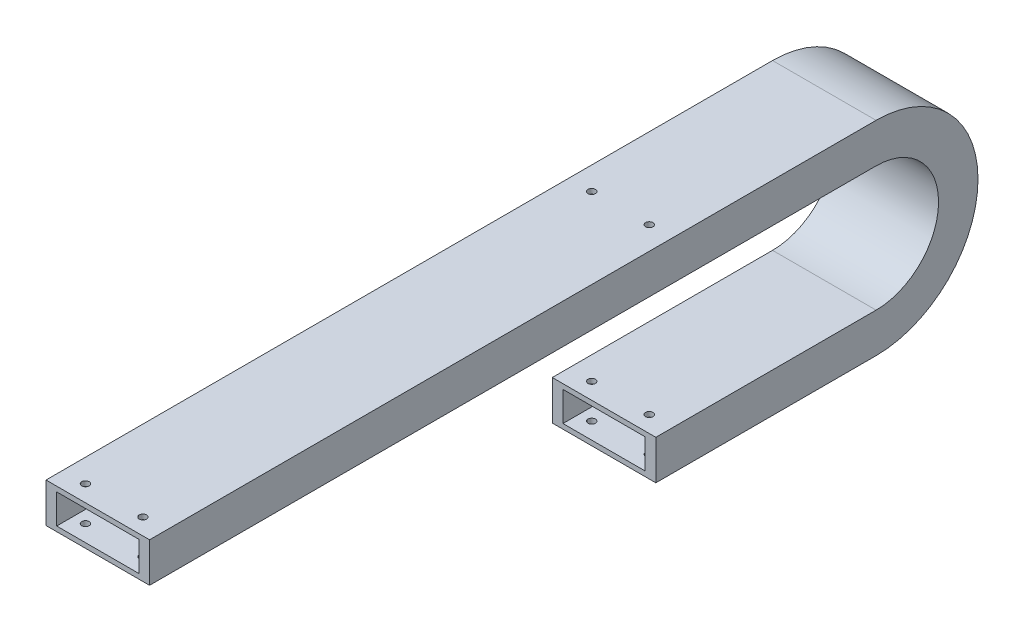
from build123d import *

# Parameters (mm, degrees)
SKETCH_1_W          = 63
SKETCH_1_H          = 24
SKETCH_1_W_2        = 50
SKETCH_1_H_2        = 18
SKETCH_5_R          = 2.25
CUT_EXTRUDE_3_DEPTH = 334.514992167


with BuildPart() as part:
    # 扫描1: sweep along a path in 草图2
    with BuildLine(Plane(origin=(0, 0, 0), x_dir=(0, 0, -1), z_dir=(1, 0, 0))) as sweep_1_path:
        Line((0, 0), (134, 0))
        ThreePointArc((134, 0), (184, 50), (134, 100))
        Line((134, 100), (-308, 100))
    # 草图1 → 扫描1 (sweep)
    with BuildSketch(Plane.XY):
        Rectangle(SKETCH_1_W, SKETCH_1_H)
        Rectangle(SKETCH_1_W_2, SKETCH_1_H_2, mode=Mode.SUBTRACT)
    sweep(path=sweep_1_path.line)

    # 草图5 → 切除-拉伸3 (cut, through all)
    with BuildSketch(Plane.XZ.offset(12)):
        with Locations((-17.5, -10)):
            Circle(SKETCH_5_R)
        with Locations((17.5, -10)):
            Circle(SKETCH_5_R)
        with Locations(Location((-17.5, 298, 0), (0, 0, 180))):
            Circle(SKETCH_5_R)
        with Locations(Location((17.5, 298, 0), (0, 0, 180))):
            Circle(SKETCH_5_R)
    extrude(amount=-CUT_EXTRUDE_3_DEPTH, mode=Mode.SUBTRACT)


solid = part.part
